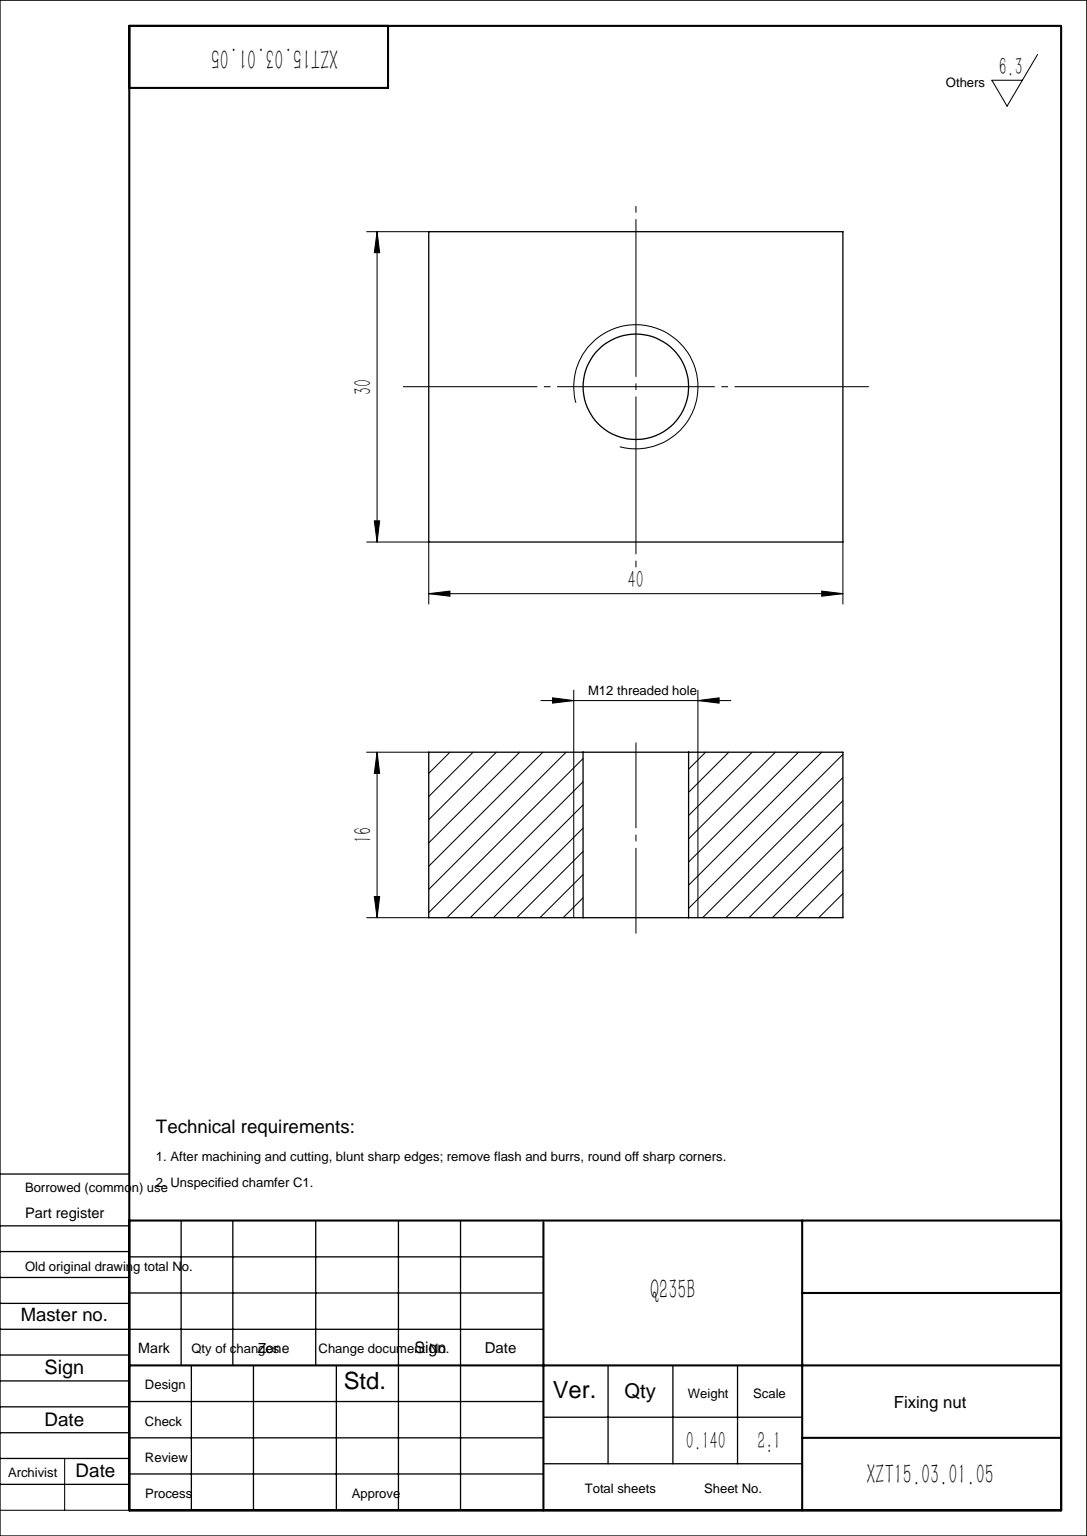
from build123d import *

# Parameters (mm, degrees)
SKETCH1_W           = 40
SKETCH1_H           = 30
BOSS_EXTRUDE1_DEPTH = 16
M12_TAPPED_HOLE1_D  = 10.2


with BuildPart() as part:
    # Sketch1 → Boss-Extrude1 (new body)
    with BuildSketch(Plane(origin=(0, 0, 0), x_dir=(1, 0, 0), z_dir=(0, 1, 0))):
        Rectangle(SKETCH1_W, SKETCH1_H)
    extrude(amount=BOSS_EXTRUDE1_DEPTH)

    # M12 Tapped Hole1 (through all)
    with Locations(Plane(origin=(0, 16, 0), x_dir=(1, 0, 0), z_dir=(0, 1, 0))):
        with Locations((0, 0)):
            Hole(M12_TAPPED_HOLE1_D / 2)


solid = part.part
